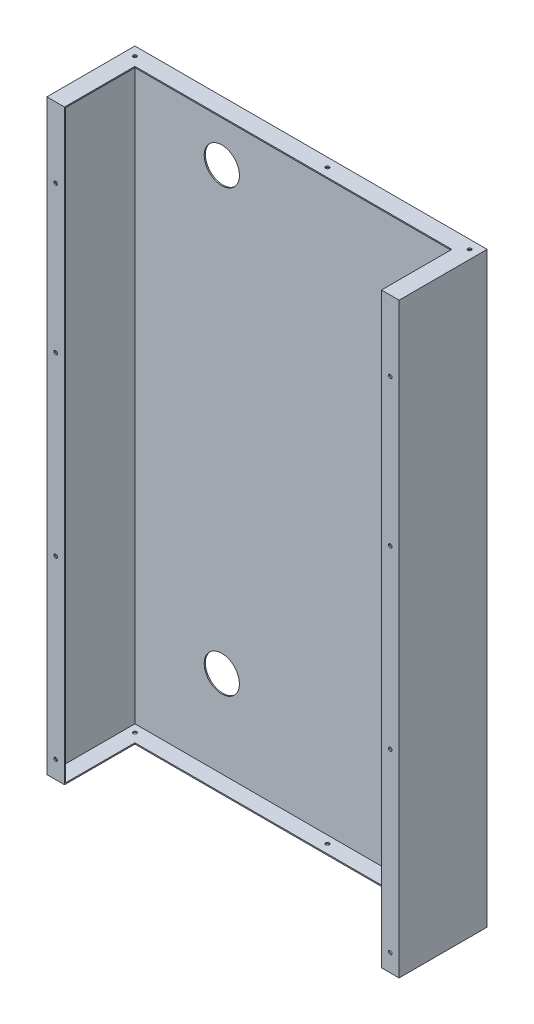
SolidWorks part; units mm, degrees
ref_plane "前视" through (0, 0, 0) normal (0, 0, 1) x (1, 0, 0)
ref_plane "上视" through (0, 0, 0) normal (0, 1, 0) x (1, 0, 0)
ref_plane "右视" through (0, 0, 0) normal (1, 0, 0) x (0, 0, -1)
sketch "草图1" plane through (0, 0, 0) normal (0, 1, 0) x (1, 0, 0)
  line L1 (0, 0) -> (600, 0)
  line L2 (0, 0) -> (0, 150)
  line L3 (0, 150) -> (600, 150)
  line L4 (600, 0) -> (600, 150)
  dimension "D1" = 150
  dimension "D2" = 600
extrude "凸台-拉伸1" add sketch "草图1" along normal blind 1000
shell "抽壳1" thickness 2
sketch "草图3" plane through (0, 0, 0) normal (0, -1, 0) x (1, 0, 0)
  line L1 (2, -148) -> (598, -148)
  line L2 (2, -148) -> (2, 0)
  line L3 (2, 0) -> (598, 0)
  line L4 (598, -148) -> (598, 0)
extrude "切除-拉伸1" cut sketch "草图3" against normal blind 400
sketch "草图4" plane through (0, 0, 0) normal (0, 0, 1) x (1, 0, 0)
  line L0 (2, 0) -> (598, 0) construction
  line L1 (2, 998) -> (30, 998)
  line L2 (2, 998) -> (2, 0)
  line L3 (2, 0) -> (30, 0)
  line L4 (30, 998) -> (30, 0)
  line L6 (598, 998) -> (570, 998)
  line L7 (598, 998) -> (598, 0)
  line L8 (598, 0) -> (570, 0)
  line L9 (570, 998) -> (570, 0)
  dimension "D1" = 28
  dimension "D2" = 28
extrude "凸台-拉伸2" add sketch "草图4" against normal blind 2
sketch "草图5" plane through (0, 0, -150) normal (0, 0, -1) x (-1, 0, 0)
  line L0 (-600, 0) -> (0, 0) construction
  line L1 (0, 1000) -> (0, 0) construction
  line L2 (-600, 1000) -> (0, 1000) construction
  circle A0 centre (-150, 150) radius 30
  circle A1 centre (-150, 900) radius 30
  dimension "D1" = 150
  dimension "D2" = 150
  dimension "D3" = 60
  dimension "D4" = 60
  dimension "D5" = 100
extrude "切除-拉伸2" cut sketch "草图5" against normal blind 2
sketch "草图6" plane through (0, 1000, 0) normal (0, 1, 0) x (1, 0, 0)
  line L0 (0, 0) -> (0, 266.5633) construction
  line L1 (0, 0) -> (787.3515, 0) construction
  line L3 (0, 150) -> (815.3779, 150) construction
  line L4 (600, 0) -> (600, 150) construction
  line L5 (30, 0) -> (570, 0)
  line L6 (30, 0) -> (30, 120)
  line L7 (30, 120) -> (570, 120)
  line L8 (570, 0) -> (570, 120)
  dimension "D1" = 30
  dimension "D2" = 30
extrude "切除-拉伸3" cut sketch "草图6" against normal blind 290
sketch "草图7" plane through (0, 0, 0) normal (0, -1, 0) x (1, 0, 0)
  line L0 (0, 0) -> (0, -150)
  line L1 (0, -150) -> (600, -150)
  line L2 (600, -150) -> (600, 0)
  line L3 (600, 0) -> (570, 0)
  line L4 (570, 0) -> (570, -120)
  line L5 (570, -120) -> (30, -120)
  line L6 (30, -120) -> (30, 0)
  line L7 (30, 0) -> (0, 0)
extrude "凸台-拉伸3" add sketch "草图7" against normal blind 2
sketch "草图8" plane through (0, 1000, 0) normal (0, 1, 0) x (1, 0, 0)
  line L0 (0, 150) -> (0, 0) construction
  line L1 (600, 0) -> (600, 150) construction
  line L3 (600, 150) -> (0, 150) construction
  circle A0 centre (15, 135) radius 3
  circle A2 centre (343, 135) radius 3
  circle A6 centre (585, 135) radius 3
  dimension "D1" = 6
  dimension "D3" = 6
  dimension "D7" = 6
  dimension "D8" = 15
  dimension "D12" = 15
  dimension "D13" = 15
  dimension "D17" = 15
  dimension "D19" = 15
extrude "切除-拉伸4" cut sketch "草图8" against normal blind 1118
sketch "草图9" plane through (0, 0, 0) normal (0, 0, 1) x (1, 0, 0)
  line L0 (15, 880) -> (15, -18.9561) construction
  line L1 (0, 1000) -> (0, 0) construction
  line L2 (0, 0) -> (30, 0) construction
  line L3 (300, 998) -> (300, 424.4888) construction
  line L4 (598, 998) -> (2, 998) construction
  circle A0 centre (15, 880) radius 3
  circle A1 centre (15, 30) radius 3
  circle A2 centre (585, 880) radius 3
  circle A3 centre (15, 330) radius 3
  circle A4 centre (585, 630) radius 3
  circle A5 centre (15, 630) radius 3
  circle A6 centre (585, 330) radius 3
  circle A7 centre (585, 30) radius 3
  dimension "D2" = 6
  dimension "D3" = 30
  dimension "D4" = 6
  dimension "D5" = 300
  dimension "D6" = 300
  dimension "D7" = 6
  dimension "D11" = 6
  dimension "D1" = 15
extrude "切除-拉伸5" cut sketch "草图9" against normal blind 10
